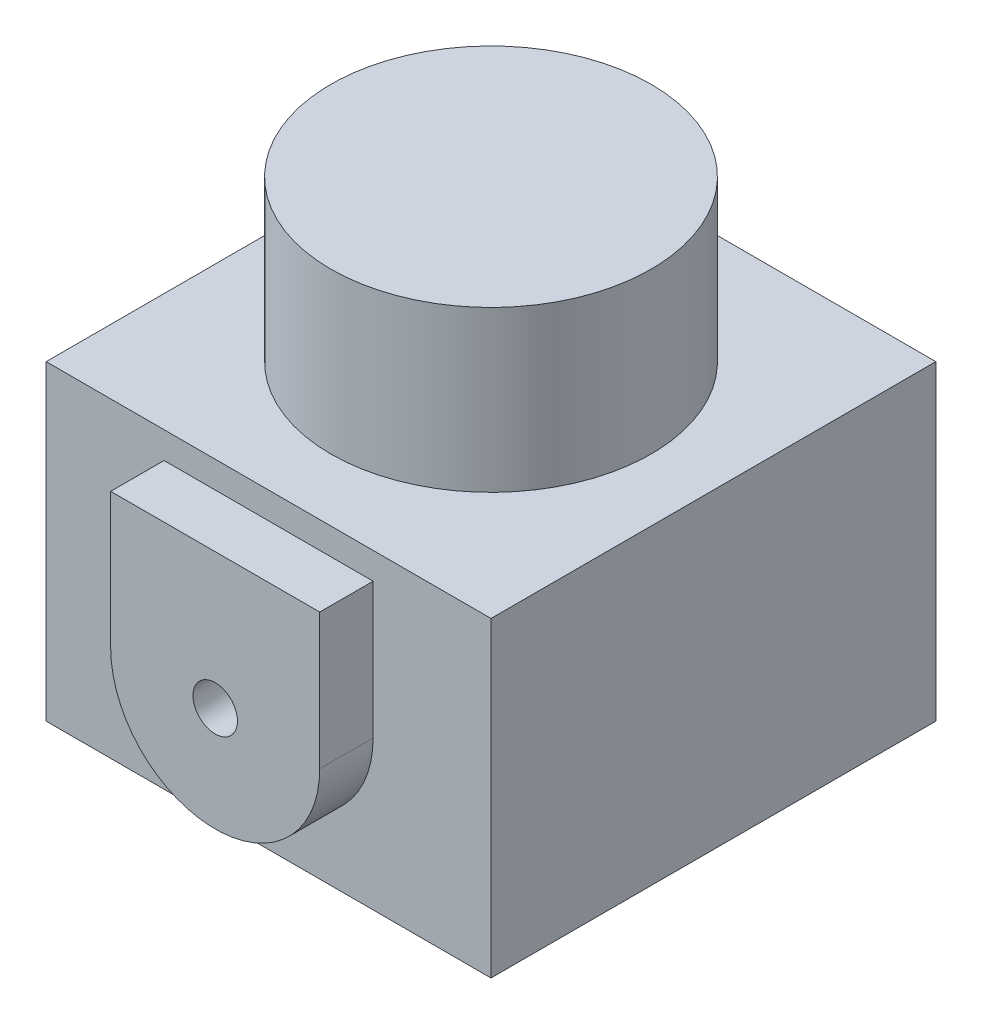
SolidWorks part; units mm, degrees
ref_plane "Front Plane" through (0, 0, 0) normal (0, 0, 1) x (1, 0, 0)
ref_plane "Top Plane" through (0, 0, 0) normal (0, 1, 0) x (1, 0, 0)
ref_plane "Right Plane" through (0, 0, 0) normal (1, 0, 0) x (0, 0, -1)
sketch "Sketch1" plane through (0, 0, 0) normal (0, 1, 0) x (1, 0, 0)
  line L1 (-25, -25) -> (25, -25)
  line L2 (-25, -25) -> (-25, 25)
  line L3 (-25, 25) -> (25, 25)
  line L4 (25, -25) -> (25, 25)
  line L5 (-25, -25) -> (25, 25) construction
  line L6 (-25, 25) -> (25, -25) construction
  point P0 (0, 0)
  dimension "D1" = 50
  dimension "D2" = 50
extrude "Boss-Extrude1" add sketch "Sketch1" along normal blind 35
sketch "Sketch2" plane through (0, 35, 0) normal (0, 1, 0) x (1, 0, 0)
  circle A0 centre (0, 0) radius 18
  dimension "D1" = 36
extrude "Boss-Extrude2" add sketch "Sketch2" along normal blind 18
sketch "Sketch3" plane through (0, 0, 25) normal (0, 0, 1) x (1, 0, 0)
  line L0 (11.75, 32) -> (-11.75, 32)
  line L2 (11.75, 32) -> (11.75, 16.75)
  line L4 (-11.75, 32) -> (-11.75, 16.75)
  line L5 (25, 35) -> (25, 0) construction
  line L6 (-25, 35) -> (25, 35) construction
  arc A0 (11.75, 16.75) -> (-11.75, 16.75) centre (0, 16.75) cw
  dimension "D3" = 11.75
  dimension "D1" = 23.5
  dimension "D2" = 15.25
  dimension "D4" = 13.25
  dimension "D5" = 3
extrude "Boss-Extrude3" add sketch "Sketch3" along normal blind 6
hole_wizard "M6 Tapped Hole1" positions "Sketch4" profile "Sketch5" tap size "M6" standard "GB"
sketch "Sketch4" plane through (0, 0, 31) normal (0, 0, 1) x (1, 0, 0)
  point P0 (0, 16.75)
sketch "Sketch5" plane through (0, 16.75, 31) normal (1, 0, 0) x (0, -1, 0)
  line L0 (0, 0) -> (0, 18.5022)
  line L1 (0, 18.5022) -> (2.5, 17)
  line L2 (2.5, 17) -> (2.5, 0)
  line L5 (2.5, 0) -> (0, 0)
  line L10 (0, 18.5022) -> (-2.5, 17) construction
  line L11 (0, -6.35) -> (0, 107.95) construction
  dimension "螺纹孔钻头直径" = 5
  dimension "螺纹孔钻头深度" = 17
  dimension "导头角度" = 118
cosmetic thread "Hole thread 1" parameters "D1"=12, "D2"=6
